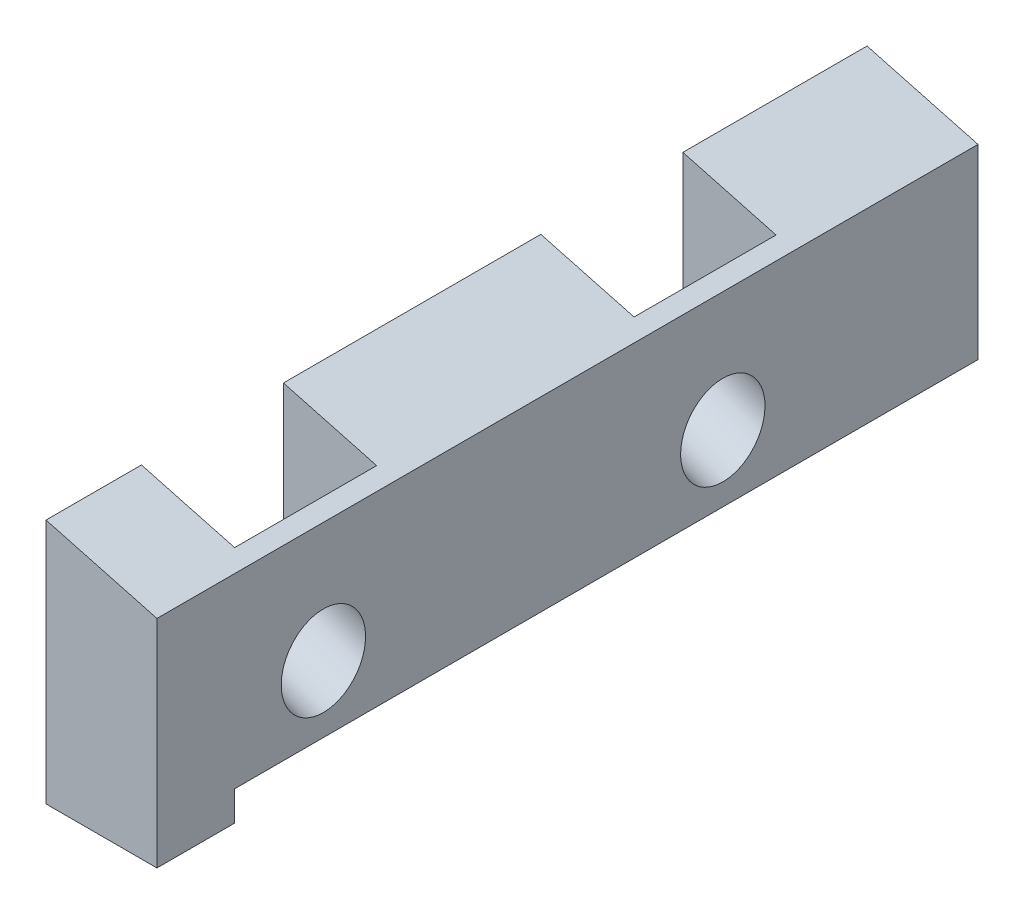
SolidWorks part; units mm, degrees
material "ZG120Mn13-2"
ref_plane "Front Plane" through (0, 0, 0) normal (0, 0, 1) x (1, 0, 0)
ref_plane "Top Plane" through (0, 0, 0) normal (0, 1, 0) x (1, 0, 0)
ref_plane "Right Plane" through (0, 0, 0) normal (1, 0, 0) x (0, 0, -1)
sketch "Sketch1" plane through (0, 0, 0) normal (0, 0, 1) x (1, 0, 0)
  line L0 (0, 0) -> (50, 13.3975)
  line L1 (50, 13.3975) -> (50, 97.3975)
  line L2 (50, 97.3975) -> (0, 110.7949)
  line L3 (0, 110.7949) -> (0, 0)
  line L4 (0, 55.3975) -> (-76.1828, 55.3975) construction
  dimension "D1" = 84
  dimension "D2" = 15
  dimension "D3" = 50
extrude "Boss-Extrude1" add sketch "Sketch1" along normal mid plane 370
sketch "Sketch2" plane through (0, 0, 185) normal (0, 0, 1) x (1, 0, 0)
  line L0 (0, 0) -> (50, 0)
  line L1 (50, 0) -> (50, 13.3975)
  line L2 (50, 13.3975) -> (0, 0)
extrude "Boss-Extrude2" add sketch "Sketch2" against normal blind 35
sketch "Sketch3" plane through (0, 0, 0) normal (0, 0, 1) x (1, 0, 0)
  line L0 (16.5173, 4.4258) -> (42.0032, 99.5402)
  line L1 (50, 13.3975) -> (0, 0) construction
  line L2 (50, 97.3975) -> (0, 110.7949) construction
  line L3 (0, 110.7949) -> (42.0032, 99.5402)
  line L4 (16.5173, 4.4258) -> (0, 0)
  line L5 (0, 0) -> (0, 110.7949)
  dimension "D1" = 15
  dimension "D2" = 17.1
extrude "Cut-Extrude1" cut sketch "Sketch3" against normal mid plane 64 from offset 110
sketch "Sketch4" plane through (0, 0, 0) normal (0, 0, 1) x (1, 0, 0)
  line L0 (16.5173, 4.4258) -> (0, 0) construction
  line L1 (0, 0) -> (0, 110.7949) construction
  line L2 (0, 110.7949) -> (42.0032, 99.5402) construction
  line L3 (16.5173, 4.4258) -> (42.0032, 99.5402) construction
  line L4 (16.5173, 4.4258) -> (0, 0)
  line L5 (0, 0) -> (0, 110.7949)
  line L6 (0, 110.7949) -> (42.0032, 99.5402)
  line L7 (16.5173, 4.4258) -> (42.0032, 99.5402)
extrude "Cut-Extrude2" cut sketch "Sketch4" against normal mid plane 64 from offset 70 offset against normal yes
sketch "Sketch7" plane through (0, 0, 0) normal (0, 0, 1) x (1, 0, 0)
  line L0 (50, 43.3975) -> (-32.7807, 43.3975) construction
  line L1 (50, 0) -> (50, 97.3975) construction
  line L2 (50, 13.3975) -> (0, 0) construction
  line L3 (50, 43.3975) -> (-23.903, 70.296)
  point P2 (50, 13.3975)
  dimension "D1" = 30
  dimension "D2" = 20
ref_plane "Plane1" through (19.7966, 54.3906, 0) normal (0.342, 0.9397, 0) x (-0.9397, 0.342, 0)
sketch "Sketch8" plane through (19.7966, 54.3906, 0) normal (0.342, 0.9397, 0) x (-0.9397, 0.342, 0)
  line L0 (-5.4253, -70) -> (95.6937, -70) construction
  line L2 (-51.9843, -51) -> (30.2017, -51)
  line L3 (30.2017, -51) -> (30.2017, -70)
  line L4 (30.2017, -70) -> (-51.9843, -70)
  line L5 (-51.9843, -51) -> (-51.9843, -70)
  dimension "D1" = 19
  dimension "D2" = 70
revolve "Cut-Revolve1" cut sketch "Sketch8" angle 360 about L0
pattern_linear "LPattern1" count 2 spacing 180 along (0, 0, 1) of "Cut-Revolve1"
